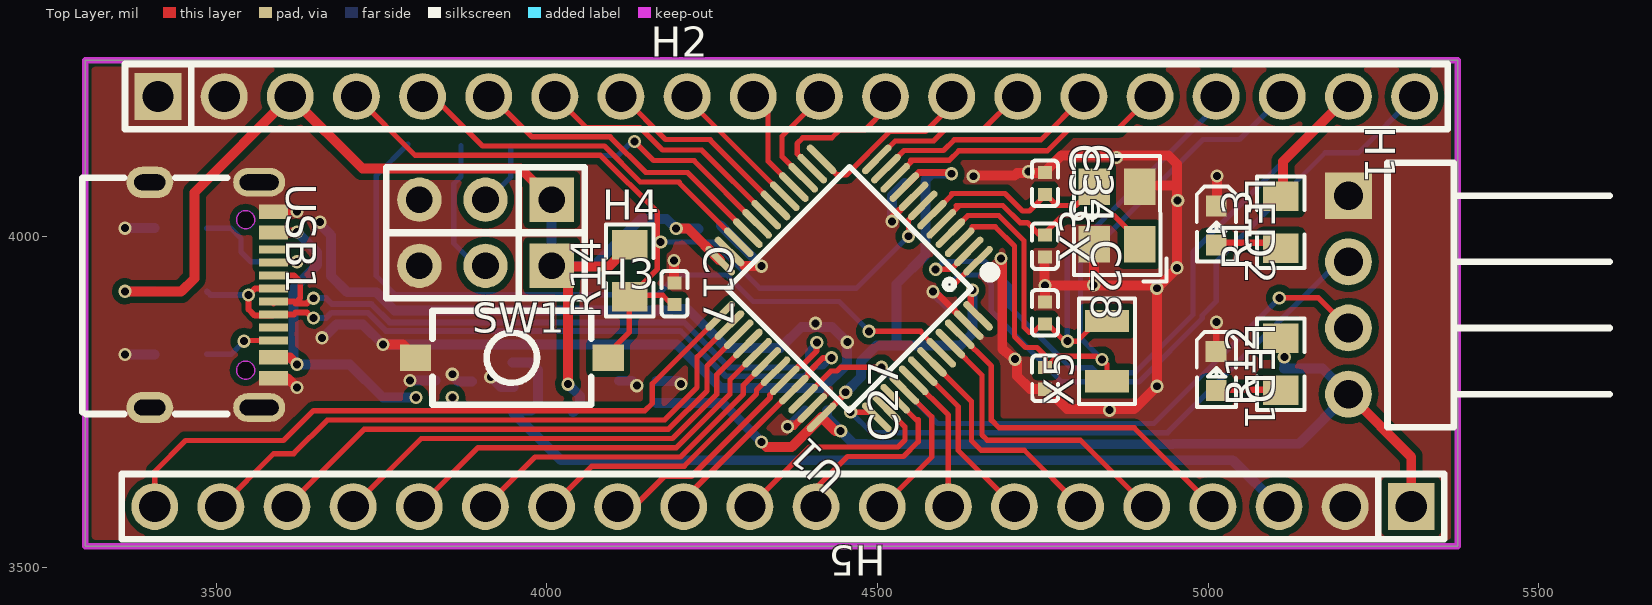
[diagram p0: Top Layer view]
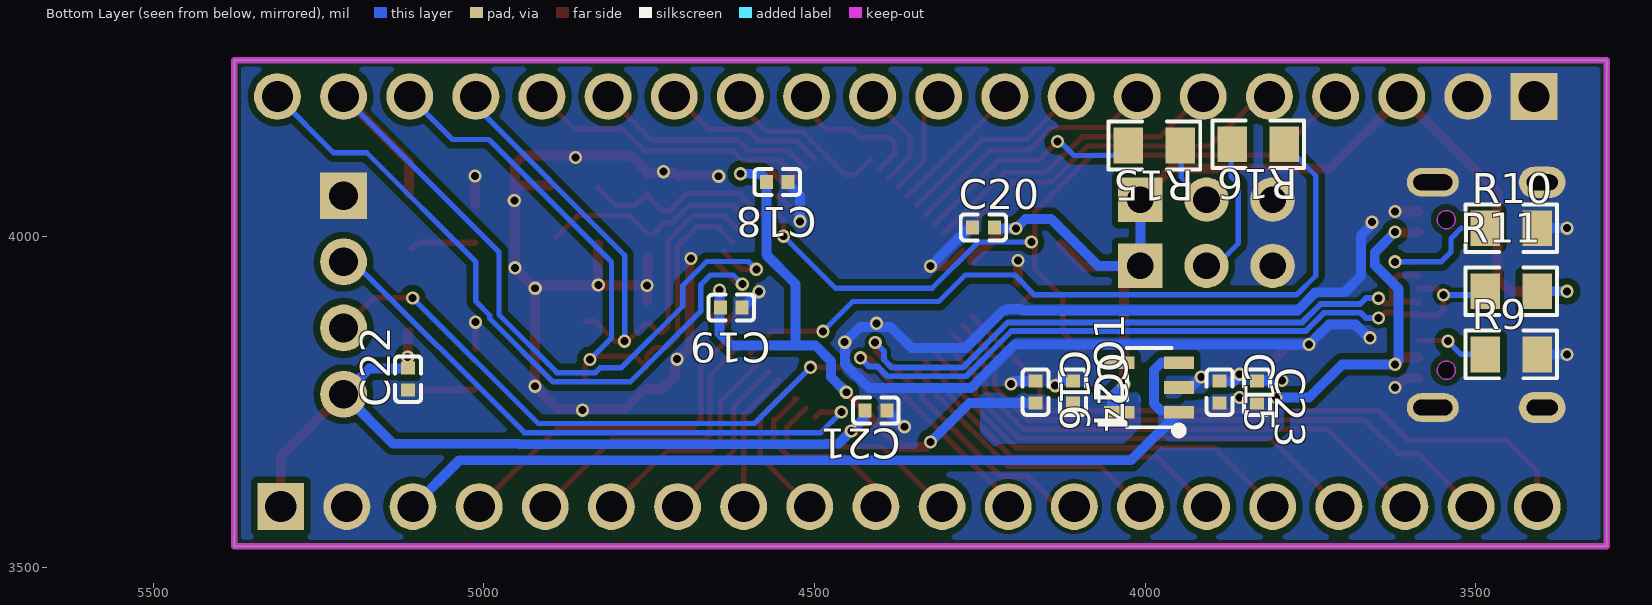
[diagram p1: Bottom Layer view, seen from below]
# Altium PCB MISC51884.pcbdoc
Units mil, origin at the board's own origin, x right, y up, seen from the top; angles counter-clockwise.
Board outline 2075 x 735 mil, 2 copper layers (Top Layer, Bottom Layer), stack 62.205 mil thick; 35 components, 49 nets, 175 pads, 64 vias.

## Layer stack, top to bottom
Top Solder Mask Layer: solder mask 0.394, Dk 3.3
Top Layer: signal copper 1.378
Dielectric1: surface 59.449, FR4, Dk 4.5
Bottom Layer: signal copper 1.378
Bottom Solder Mask Layer: solder mask 0.394, Dk 3.3

## Board outline
3301.94,4266.99 3301.94,3531.99 5376.94,3531.99 5376.94,4266.99

## Design rules (kind name [scope] priority, off if disabled: settings)
BoardOutlineClearance copperThickness2oz_1 [All] p2 off: genericclearance=7.99 ignorepadtopadclearanceinfootprint=FALSE except(0: Arc-SplitContinuation Track-SplitContinuation SMDPad-SplitContinuation THPad-SplitContinuation Via-SplitContinuation Fill-SplitContinuation Region-SplitContinuation Poly-SplitContinuation Text-SplitContinuation Hole-SplitContinuation; 5.98: Arc-CutoutEdge SMDPad-CutoutEdge THPad-CutoutEdge Via-CutoutEdge Fill-CutoutEdge Region-CutoutEdge Text-CutoutEdge; 6.93: Hole-OutlineEdge Hole-CutoutEdge; 10: Poly-OutlineEdge Poly-CutoutEdge; 11.81: Arc-OutlineEdge Track-OutlineEdge SMDPad-OutlineEdge THPad-OutlineEdge Via-OutlineEdge Fill-OutlineEdge Region-OutlineEdge Text-OutlineEdge Track-CutoutEdge)
BoardOutlineClearance safeClearance1_1 [All] p4: genericclearance=6 ignorepadtopadclearanceinfootprint=FALSE except(0: Arc-SplitContinuation Track-SplitContinuation SMDPad-SplitContinuation THPad-SplitContinuation Via-SplitContinuation Fill-SplitContinuation Region-SplitContinuation Poly-SplitContinuation Text-SplitContinuation Hole-SplitContinuation; 6: Arc-CutoutEdge Track-CutoutEdge SMDPad-CutoutEdge THPad-CutoutEdge Via-CutoutEdge Fill-CutoutEdge Region-CutoutEdge Text-CutoutEdge Hole-CutoutEdge; 10: Poly-OutlineEdge Poly-CutoutEdge; 11.8: Arc-OutlineEdge Track-OutlineEdge SMDPad-OutlineEdge THPad-OutlineEdge Via-OutlineEdge Fill-OutlineEdge Region-OutlineEdge Text-OutlineEdge Hole-OutlineEdge)
BoardOutlineClearance copperThickness1oz_1 [All] p6: genericclearance=6 ignorepadtopadclearanceinfootprint=FALSE except(0: Arc-SplitContinuation Track-SplitContinuation SMDPad-SplitContinuation THPad-SplitContinuation Via-SplitContinuation Fill-SplitContinuation Region-SplitContinuation Poly-SplitContinuation Text-SplitContinuation Hole-SplitContinuation; 6: Track-CutoutEdge SMDPad-CutoutEdge THPad-CutoutEdge Via-CutoutEdge Text-CutoutEdge; 6.93: Hole-OutlineEdge Hole-CutoutEdge; 10: Poly-OutlineEdge Poly-CutoutEdge; 11.8: Arc-OutlineEdge Track-OutlineEdge SMDPad-OutlineEdge THPad-OutlineEdge Via-OutlineEdge Fill-OutlineEdge Region-OutlineEdge Text-OutlineEdge Fill-CutoutEdge Region-CutoutEdge; 11.81: Arc-CutoutEdge)
Clearance copperThickness2oz [All] p1 off: gap=7.99 ignorepadtopadclearanceinfootprint=FALSE except(5.98: SMDPad-Track SMDPad-SMDPad THPad-Track SMDPad-THPad THPad-THPad Track-Via SMDPad-Via THPad-Via Via-Via Fill-Track Region-Track Fill-SMDPad Region-SMDPad Fill-THPad Region-THPad Fill-Via Region-Via Fill-Fill Fill-Region Region-Region Arc-Track Arc-SMDPad Arc-THPad Arc-Via Fill-Arc Region-Arc Arc-Arc Text-Track SMDPad-Text Text-THPad Text-Via Fill-Text Region-Text Arc-Text Text-Text; 6.93: Hole-Track Hole-SMDPad Hole-THPad Hole-Via Fill-Hole Region-Hole Hole-Arc Hole-Text; 10: Poly-Track Poly-SMDPad Poly-THPad Poly-Via Poly-Fill Poly-Region Poly-Poly Poly-Arc Poly-Text Poly-Hole)
Clearance safeClearance1 [(InNet('USB_D-_PA11')) vs (InNet('GND'))] p3: gap=6 ignorepadtopadclearanceinfootprint=FALSE except(10: Poly-Arc Poly-Text Poly-Hole)
Clearance copperThickness1oz [All] p5: gap=6 ignorepadtopadclearanceinfootprint=FALSE except(5.98: SMDPad-Track SMDPad-SMDPad THPad-Track SMDPad-THPad THPad-THPad Track-Via SMDPad-Via THPad-Via Via-Via Fill-SMDPad Region-SMDPad Fill-THPad Region-THPad Fill-Via Region-Via Fill-Fill Fill-Region Region-Region; 6.93: Hole-Track Hole-SMDPad Hole-THPad Hole-Via Fill-Hole Region-Hole Hole-Arc Hole-Text; 10: Poly-Track Poly-SMDPad Poly-THPad Poly-Via Poly-Fill Poly-Region Poly-Poly Poly-Arc Poly-Text Poly-Hole; 11.8: Fill-Track Region-Track)
DiffPairsRouting differentialPair [All] p1: maxlimit=6 minlimit=6 mostfreqgap=6 toplayer_minwidth=5 toplayer_prefwidth=9 toplayer_maxwidth=100 toplayer_mingap=4 toplayer_prefgap=5 toplayer_maxgap=5 bottomlayer_minwidth=5 bottomlayer_prefwidth=9 bottomlayer_maxwidth=100 bottomlayer_mingap=4 bottomlayer_prefgap=5 bottomlayer_maxgap=5 maxuncoupledlength=1000
HoleToHoleClearance otherClearance [All] p1: gap=11.81 allowstackedmicrovias=TRUE
Length netLength [All] p1: minlimit=0 maxlimit=0
MatchedLengths netLengthTolerance [All] p1: tolerance=1000
PasteMaskExpansion pasteMaskExpansion [All] p1: expansion=0
PlaneConnect innerPlane [All] p1: planeconnectstyle=Relief reliefexpansion=20 reliefentries=4 reliefconductorwidth=10 reliefairgap=10
PolygonConnect "copperRegion_Top Layer" [(InNet('GND')) And OnLayer('Top Layer')] p1: connectstyle=Direct reliefconductorwidth=10 reliefentries=4 polygonreliefangle="90 Angle" airgapwidth=10 via.connectstyle=Relief via.reliefconductorwidth=10 via.reliefentries=4 via.polygonreliefangle="90 Angle" via.airgapwidth=10
PolygonConnect "copperRegion_Bottom Layer" [(InNet('GND')) And OnLayer('Bottom Layer')] p2: connectstyle=Direct reliefconductorwidth=10 reliefentries=4 polygonreliefangle="90 Angle" airgapwidth=10 via.connectstyle=Relief via.reliefconductorwidth=10 via.reliefentries=4 via.polygonreliefangle="90 Angle" via.airgapwidth=10
PolygonConnect copperRegion [(InNet('GND'))] p3: connectstyle=Direct reliefconductorwidth=10 reliefentries=4 polygonreliefangle="90 Angle" airgapwidth=10 via.connectstyle=Relief via.reliefconductorwidth=10 via.reliefentries=4 via.polygonreliefangle="90 Angle" via.airgapwidth=10
RoutingVias viaSize [All] p1: holewidth=12 width=20 viastyle="Through Hole" minholewidth=11.81 minwidth=19.68 maxholewidth=248.03 maxwidth=393.7
SolderMaskExpansion solderMaskExpansion [IsVia] p1: expansion=-1000 istentingtop=TRUE
SolderMaskExpansion solderMaskExpansion [All] p2: expansion=2 istentingtop=FALSE
Width pwr [(InNet('+5V') OR InNet('GND') OR InNet('3V3'))] p1: maxlimit=10 minlimit=10 preferedwidth=10 toplayer_minwidth=5 toplayer_maxwidth=100 toplayer_prefwidth=15 bottomlayer_minwidth=5 bottomlayer_maxwidth=100 bottomlayer_prefwidth=15
Width copperThickness1oz_2 [All] p2: maxlimit=10 minlimit=10 preferedwidth=10 toplayer_minwidth=5 toplayer_maxwidth=100 toplayer_prefwidth=8 bottomlayer_minwidth=5 bottomlayer_maxwidth=100 bottomlayer_prefwidth=8

## Components (designator, comment, footprint, x,y, rotation, side; value= is the part's Value field where it differs from the comment)
C15 "100nF" C0402 3887.18,3765.13 r270 bottom
C16 "100nF" C0402 4165.39,3765.13 r270 bottom
C17 "100nF" C0402 4192.92,3913.82 r270 top
C18 "100nF" C0402 4556.15,4082.72 r0 bottom
C19 "100nF" C0402 4625.75,3892.7 r0 bottom
C20 "100nF" C0402 4244.28,4014.21 r180 bottom
C21 "100nF" C0402 4406.94,3736.99 r0 bottom
C22 "100nF" C0402 5114.29,3784.59 r90 bottom
C23 "1uF" C0402 3830.97,3765.13 r270 bottom
C24 "1uF" C0402 4109.18,3765.13 r270 bottom
C27 "12pF" C0402 4753.42,3785.9 r90 top
C28 "12pF" C0402 4752.88,3884.91 r270 top
C33 "12pF" C0402 4752.85,4080.7 r270 top
C34 "12pF" C0402 4752.85,3985.84 r270 top
H1 "DZ254W-11-04-65" HDR-TH_4P-P2.54-H-M-W10.3 5211.94,3911.99 r270 top
H2 "2.54-1*20P直针" HDR-TH_20P-P2.54-V-M-1 4361.94,4211.99 r0 top
H3 "PZ254V-11-03P" HDR-TH_3P-P2.54-V-M_PZ254V-11-03P 3907.09,3955.98 r180 top
H4 "PZ254V-11-03P" HDR-TH_3P-P2.54-V-M_PZ254V-11-03P 3907.09,4055.98 r180 top
H5 "2.54-1*20P直针" HDR-TH_20P-P2.54-V-M-1 4356.94,3591.99 r180 top
LDO1 "ME6211C33M5G-N" SOT-23-5_L3.0-W1.7-P0.95-LS2.8-BL 3993.82,3771.99 r90 bottom
LED1 "NCD0603R1" LED0603-RD_RED 5011.94,3796.99 r270 top
LED2 "NCD0603B1" LED0603-RD 5011.94,4016.99 r270 top
R9 "5.1kΩ" R0805 3446.31,3822.08 r180 bottom
R10 "5.1kΩ" R0805 3446.31,4012.89 r180 bottom
R11 "1.5kΩ" R0805 3446.31,3917.48 r180 bottom
R12 "1kΩ" R0805 5109.57,3807.13 r90 top
R13 "1kΩ" R0805 5109.57,4021.85 r90 top
R14 "10kΩ" R0805 4125.3,3948.81 r90 top
R15 "10kΩ" R0805 3985.86,4138.03 r0 bottom
R16 "10kΩ" R0805 3829.01,4139.92 r0 bottom
SW1 "TS-1101-B-W" KEY-SMD_2P-L6.0-W3.6-P7.4-LS8.0-L 3946.94,3816.99 r0 top
U1 "STM32F103C8T6" LQFP-48_L7.0-W7.0-P0.50-LS9.0-BL 4456.94,3921.99 r135 top
USB1 "TYPE-C 16PIN 2MD(073)" USB-C-SMD_TYPE-C-6PIN-2MD-073 3493.04,3911.99 r270 top
X3 "8MHz" CRYSTAL-SMD_4P-L3.2-W2.5-BL-1 4861.94,4031.99 r90 top
X5 "32.768kHz" OSC-SMD_L3.2-W1.5 4846.94,3826.99 r90 top

## Footprints (in the part's own frame and the unit in brackets; to place one, negate y for a bottom-side part, rotate by r counter-clockwise, add the part's x,y. Pads: shape width x height; smd on the part's side, far side on the other; paste and mask are expansions set on the pad)
C0402 [mm]
  rect 0.5x0.54 smd: 1(-0.42,0) 2(0.42,0)
  silkscreen extent -0.87,-0.5 0.87,0.5
CRYSTAL-SMD_4P-L3.2-W2.5-BL-1 [mm]
  rect 1.4x1.2 smd: 1(-1.1,-0.875) 2(1.1,-0.875) 3(1.1,0.875) 4(-1.1,0.875)
  silkscreen extent -2.54,-1.9 2.29,1.65
HDR-TH_3P-P2.54-V-M_PZ254V-11-03P [mm]
  rect 1.7x1.7 hole 1.02: 1(-2.54,0)
  round 1.7 hole 1.02: 2(0,0) 3(2.54,0)
  silkscreen extent -3.81,-1.25 3.81,1.25
HDR-TH_4P-P2.54-H-M-W10.3 [mm]
  rect 1.8x1.8 hole 1.1: 1(-3.81,0)
  round 1.8 hole 1.1: 2(-1.27,0) 3(1.27,0) 4(3.81,0)
  silkscreen extent -5.08,1.5 5.08,10.04
HDR-TH_20P-P2.54-V-M-1 [mm]
  rect 1.8x1.8 hole 1.2: 1(-24.13,0)
  round 1.8 hole 1.2: 2(-21.59,0) 3(-19.05,0) 4(-16.51,0) 5(-13.97,0) 6(-11.43,0) 7(-8.89,0) 8(-6.35,0) 9(-3.81,0) 10(-1.27,0) 11(1.27,0) 12(3.81,0) 13(6.35,0) 14(8.89,0) 15(11.43,0) 16(13.97,0) 17(16.51,0) 18(19.05,0) 19(21.59,0) 20(24.13,0)
  silkscreen extent -25.4,-1.25 25.4,1.25
KEY-SMD_2P-L6.0-W3.6-P7.4-LS8.0-L [mm]
  rect 1.2x1 smd: 1(-3.7,0) 2(3.7,0)
  silkscreen extent -3.05,-1.8 3.05,1.8
LED0603-RD [mm]
  rect 0.8x0.8 smd: 1(-0.749,0) 2(0.749,0)
  silkscreen extent -1.49,-0.75 1.39,0.76
LED0603-RD_RED [mm]
  rect 0.8x0.8 smd: 1(-0.749,-0.003) 2(0.749,0.003)
  silkscreen extent -1.49,-0.75 1.39,0.76
LQFP-48_L7.0-W7.0-P0.50-LS9.0-BL [mm]
  oval 0.27x1.5 smd paste+0 mask+0.05: 1(-2.75,-4.25) 2(-2.25,-4.25) 3(-1.75,-4.25) 4(-1.25,-4.25) 5(-0.75,-4.25) 6(-0.25,-4.25) 7(0.25,-4.25) 8(0.75,-4.25) 9(1.25,-4.25) 10(1.75,-4.25) 11(2.25,-4.25) 12(2.75,-4.25) 25(2.75,4.25) 26(2.25,4.25) 27(1.75,4.25) 28(1.25,4.25) 29(0.75,4.25) 30(0.25,4.25) 31(-0.25,4.25) 32(-0.75,4.25) 33(-1.25,4.25) 34(-1.75,4.25) 35(-2.25,4.25) 36(-2.75,4.25)
  oval 1.5x0.27 smd paste+0 mask+0.05: 13(4.25,-2.75) 14(4.25,-2.25) 15(4.25,-1.75) 16(4.25,-1.25) 17(4.25,-0.75) 18(4.25,-0.25) 19(4.25,0.25) 20(4.25,0.75) 21(4.25,1.25) 22(4.25,1.75) 23(4.25,2.25) 24(4.25,2.75) 37(-4.25,2.75) 38(-4.25,2.25) 39(-4.25,1.75) 40(-4.25,1.25) 41(-4.25,0.75) 42(-4.25,0.25) 43(-4.25,-0.25) 44(-4.25,-0.75) 45(-4.25,-1.25) 46(-4.25,-1.75) 47(-4.25,-2.25) 48(-4.25,-2.75)
  silkscreen extent -3.59,-4.46 3.3,3.34
OSC-SMD_L3.2-W1.5 [mm]
  rect 0.85x1.7 smd: 1(-1.155,0) 2(1.155,0)
  silkscreen extent -2.03,-1.08 2.03,1.08
R0805 [mm]
  rect 1.133x1.377 smd paste-100 mask+0.051: 1(-1,0) 2(1,0)
  silkscreen extent -1.76,-0.92 1.76,0.92
SOT-23-5_L3.0-W1.7-P0.95-LS2.8-BL [mm]
  rect 0.49x1.157 smd: 1(-0.95,-1.154) 2(0,-1.154) 3(0.95,-1.154)
  rect 0.49x1.175 smd: 4(0.95,1.154) 5(-0.95,1.154)
  silkscreen extent -1.8,-1.29 1.53,0.85
USB-C-SMD_TYPE-C-6PIN-2MD-073 [mm]
  rect 0.55x1.1 smd paste-100 mask+0.05: 1(-3.2,2.375) 2(-2.4,2.375) 11(2.4,2.375) 12(3.2,2.375)
  rect 0.3x1.1 smd paste-100 mask+0.05: 3(-1.75,2.375) 4(-1.25,2.375) 5(-0.75,2.375) 6(-0.25,2.375) 7(0.25,2.375) 8(0.75,2.375) 9(1.25,2.375) 10(1.75,2.375)
  oval 1.2x1.8 hole 0.6 slot 1.2 at 90 deg paste+0 mask+0.05: 13(-4.325,-2.375) 14(4.325,-2.375)
  oval 1.1x2 hole 0.6 slot 1.5 at 90 deg paste+0 mask+0.05: 13(-4.325,1.825) 14(4.325,1.825)
  Board Outline Layer circle w0.003: c-2.89,1.305 r0.35
  Board Outline Layer circle w0.003: c2.89,1.305 r0.35
  Board Outline Layer region: -2.89,1.655 -2.738,1.62 -2.616,1.523 -2.549,1.383 -2.549,1.227 -2.616,1.087 -2.738,0.99 -2.89,0.955 -2.89,0.955 -3.042,0.99 -3.164,1.087 -3.231,1.227 -3.231,1.383 -3.164,1.523 -3.042,1.62 -2.89,1.655
  Board Outline Layer region: -2.89,1.655 -2.812,1.646 -2.738,1.62 -2.672,1.579 -2.616,1.523 -2.575,1.457 -2.549,1.383 -2.54,1.305 -2.549,1.227 -2.575,1.153 -2.616,1.087 -2.672,1.031 -2.738,0.99 -2.812,0.964 -2.89,0.955 -2.968,0.964 -3.042,0.99 -3.108,1.031 -3.164,1.087 -3.205,1.153 -3.231,1.227 -3.24,1.305 -3.231,1.383 -3.205,1.457 -3.164,1.523 -3.108,1.579 -3.042,1.62 -2.968,1.646
  Board Outline Layer region: 2.89,1.655 3.042,1.62 3.164,1.523 3.231,1.383 3.231,1.227 3.164,1.087 3.042,0.99 2.89,0.955 2.89,0.955 2.738,0.99 2.616,1.087 2.549,1.227 2.549,1.383 2.616,1.523 2.738,1.62 2.89,1.655
  Board Outline Layer region: 2.89,1.655 2.968,1.646 3.042,1.62 3.108,1.579 3.164,1.523 3.205,1.457 3.231,1.383 3.24,1.305 3.231,1.227 3.205,1.153 3.164,1.087 3.108,1.031 3.042,0.99 2.968,0.964 2.89,0.955 2.812,0.964 2.738,0.99 2.672,1.031 2.616,1.087 2.575,1.153 2.549,1.227 2.54,1.305 2.549,1.383 2.575,1.457 2.616,1.523 2.672,1.579 2.738,1.62 2.812,1.646
  Multi-Layer board cut-out: -2.89,1.655 -2.738,1.62 -2.616,1.523 -2.549,1.383 -2.549,1.227 -2.616,1.087 -2.738,0.99 -2.89,0.955 -2.89,0.955 -3.042,0.99 -3.164,1.087 -3.231,1.227 -3.231,1.383 -3.164,1.523 -3.042,1.62 -2.89,1.655
  Multi-Layer board cut-out: 2.89,1.655 3.042,1.62 3.164,1.523 3.231,1.383 3.231,1.227 3.164,1.087 3.042,0.99 2.89,0.955 2.89,0.955 2.738,0.99 2.616,1.087 2.549,1.227 2.549,1.383 2.616,1.523 2.738,1.62 2.89,1.655
  silkscreen extent -4.5,-4.97 4.57,0.6

## Via types
v1: diameter 20, hole 12, Top Layer to Bottom Layer, 64 vias

## Nets (pads, with @x,y where several pads share a name; then routed paths per layer and width w, separated by ;. In a path a pad name is that pad's centre, name@x,y a point inside that pad or via, vN(x,y) a via of type N, cw(c..) or ccw(c..) an arc to the next point about the centre after c; other vN are vias at no path point)
3V3: C16.2 C18.2 C19.2 C20.2 C21.2 C22.2 C24.2 H1.4 H2.3 H3.1 H4.1 H5.1 LDO1.5 R11.2 R12.2 R14.2 U1.9 U1.24 U1.36 U1.48 | length 4121
  Top Layer w10: U1.36 v1@4451.7,3763.64 ; U1.9 4562.45,4097.09 ; 4562.22,4097.09 4562.45,4097.09 ; v1(4611.86,4095.24) 4610.01,4097.09 4562.45,4097.09 ; v1(4643.5,3919.17) 4641.01,3916.68 4641.01,3891.04 U1.48
  Top Layer w15: v1(3361.94,3917.48) 3362.43,3916.99 3446.94,3916.99 3466.94,3936.99 3466.94,4066.99 H2.3 3721.01,4102.93 3960.14,4102.93 H4.1 ; H3.1 4031.94,3931.12 v1(4031.94,3776.99) ; H3.1@4010.18,3955.18 4093.96,3955.18 R14.2@4126.94,3988.16 ; v1(4195.4,4012.55) 4213.27,4012.55 U1.24 ; v1(4324.44,3689.49) 4331.94,3681.99 4370.06,3681.99 U1.36 4436.01,3706.3 v1(4444.17,3706.3) ; R12.2@5113.38,3856.18 5114.92,3854.64 v1(5114.92,3818.06) ; H1.4 5306.94,3667 H5.1
  Bottom Layer w15: v1(3361.94,3917.48) R11.2 ; H4.1 H3.1 4070.93,3955.98 4141.94,4026.99 4180.96,4026.99 v1(4195.4,4012.55) 4228.31,4012.55 C20.2@4229.39,4011.47 ; v1(4031.94,3776.99) 4049.84,3759.09 4049.84,3745.2 LDO1.5 ; C16.2 4265.34,3748.59 v1(4324.44,3689.49) ; C21.2 4423.48,3726.99 v1(4444.17,3706.3) 4463.48,3686.99 4482.23,3686.99 4483.05,3686.18 4945.87,3686.18 4946.69,3686.99 5136.94,3686.99 H1.4@5211.68,3761.73 ; v1(4451.7,3764.78) 4474.82,3787.9 4474.82,3811.66 4498.54,3835.39 4528.57,3835.39 ; C18.2 4572.69,3972.74 4528.57,3928.62 4528.57,3835.39 ; C18.2@4573.09,4087 4581.34,4095.24 v1(4611.86,4095.24) ; v1(4643.5,3919.17) C19.2@4643.5,3894.17 ; C19.2@4643.7,3893.97 C19.2@4643.5,3894.17 ; C22.2@5114.15,3800.69 5172.73,3800.69 H1.4@5211.68,3761.73 ; C22.2@5114.92,3805.31 v1(5114.92,3818.06) ; H1.4 H1.4@5211.68,3761.73 ; 4528.57,3835.39 4625.33,3835.39 4643.5,3853.56 C19.2@4643.5,3894.17
$1N141: R9.1 USB1.10 | length 109.6
  Top Layer w8: v1(3541.94,3841.99) 3543.04,3843.09 USB1.10
  Bottom Layer w8: R9.1 3522.02,3822.08 v1(3541.94,3841.99)
$1N146: R10.1 USB1.4 | length 205
  Top Layer w8: USB1.4 3587.34,3961.99 v1(3621.94,3961.99)
  Bottom Layer w8: R10.1 3521.94,4012.89 3537.39,3997.44 3537.39,3976.99 3552.39,3961.99 v1(3621.94,3961.99)
$1N157: LED1.2 R12.1 | length 96.1
  Top Layer w10: LED1.2@5015.31,3768.32 5107.02,3768.32 R12.1@5110.11,3771.4
$1N159: LED2.2 R13.1 | length 98.3
  Top Layer w10: LED2.2@5013,3990.86 5099.32,3990.86 R13.1@5107.79,3982.38
$1N169: H3.2 R16.2 | length 216
  Bottom Layer w8: R16.2@3870.17,4137.87 3870.17,4091.2 3859.01,4080.04 3859.01,3989.74 3896.55,3952.2 H3.2@3906.7,3952.2
$1N174: H4.2 R15.1 | length 98.3
  Bottom Layer w8: H4.2@3908.72,4053.66 3945.25,4090.19 R15.1@3945.25,4136.86
+5V: C15.2 C23.2 H5.3 LDO1.1 LDO1.3 USB1.2 USB1.11 | length 1856.5
  Top Layer w15: USB1.11 3611.43,3817.5 v1(3621.92,3807.01) ; USB1.2 3621.43,4006.48 v1(3621.94,4006.99)
  Bottom Layer w15: v1(3621.94,4006.99) 3652.63,3976.3 3652.63,3956.99 3616.94,3921.3 3616.94,3811.99 v1(3621.92,3807.01) 3701.92,3807.01 3751.94,3756.99 v1(3801.94,3756.99) ; LDO1.3@3947.88,3809.85 3975.29,3809.85 3986.58,3798.56 3986.58,3747.5 3975.97,3736.9 3952.33,3736.9 LDO1.1@3952.18,3736.76 ; LDO1.1 4021,3661.99 5036.94,3661.99 H5.3
  other v1: 3856.94,3756.99
BOOT0: R16.1 U1.44 | length 1147.8
  Top Layer w8: v1(4486.94,3856.99) 4565.64,3856.99 ; 4563.7,3856.99 U1.44
  Bottom Layer w8: R16.1 3741.94,4092.22 3741.94,3941.04 3770.83,3912.14 4167.09,3912.14 4196.94,3941.99 4271.94,3941.99 4311.94,3901.99 4441.94,3901.99 v1(4486.94,3856.99)
BOOT1: R15.2 U1.20 | length 347
  Top Layer w8: v1(4132.44,4144.03) 4161.3,4115.16 4222.94,4115.16 ; 4222,4115.16 U1.20
  Bottom Layer w8: R15.2@4031.49,4122.65 4107.59,4122.65 v1@4130.93,4145.99
GND: C15.1 C16.1 C17.1 C18.1 C19.1 C20.1 C21.1 C22.1 C23.1 C24.1 C27.1 C28.1 C33.1 C34.2 H1.1 H2.1 H2.2 H3.3 H4.3 H5.2 LDO1.2 LED1.1 LED2.1 R9.2 R10.2 SW1.1 U1.8 U1.23 U1.35 U1.47 USB1.1 USB1.12 USB1.13 USB1.14 X3.2 X3.4 | length 4271.5
  Top Layer w10: U1.23 4298.14,3955.52 ; v1@4364.3,3712.81 v1@4373.54,3712.81 ; v1@4373.03,3712.81 U1.35 ; v1@4521.86,4023.23 v1@4521.86,4031.08 ; v1@4521.86,4028.67 U1.8 ; v1@4583.15,3917.71 v1@4586.39,3917.71 ; v1@4586.49,3917.71 U1.47 ; LED1.1@5012.23,3830.74 v1(5012.23,3870.82)
  Top Layer w15: USB1.12 3607.92,3786.01 v1(3621.94,3771.99) ; USB1.1 v1(3621.94,4037.98) ; v1(3751.94,3836.99) 3782.47,3836.99 SW1.1@3801.31,3818.15 ; C17.1@4192,3931.79 v1(4192,3963.87) ; 4298.56,3955.52 v1@4324.45,3955.52 ; v1@4645.01,4092.55 4707.28,4092.55 4710.98,4096.24 C33.1@4752.9,4096.24 ; v1(4686.7,3966.89) 4688.47,3965.13 4688.47,3830.37 v1@4708.9,3813.81 ; v1(4707.91,3814.81) v1@4708.9,3813.81 ; C34.2@4752.52,3966.86 4752.52,3927.67 v1@4753.4,3926.79 ; C28.1@4752.96,3903 v1(4752.96,3926.34) v1@4926.93,3926.34 ; C33.1@4753.52,4098.71 4777.7,4122.89 4939.95,4122.89 4952.9,4109.94 v1@4952.9,3953.02 ; C27.1@4754.84,3770.03 4730.56,3770.03 4710.99,3789.61 4710.99,3811.73 v1@4708.9,3813.81 ; C27.1@4759.16,3766.79 4786.54,3739.41 4887.96,3739.41 v1(4922.43,3773.88) 4922.21,3774.1 v1(4922.21,3922.08) ; v1@4827.03,3927.54 X3.4@4827.03,3988.24 ; X3.2@4899.86,4077.25 4947.06,4077.25 4952.46,4082.65 ; v1@4922.66,3922.07 v1@4926.93,3926.34 ; v1@4953.48,3951.58 4952.16,3951.58 v1@4926.93,3926.34 ; LED2.1@5013,4049.43 v1(5013,4091.82)
  Bottom Layer w15: v1(3361.94,3822.08) R9.2 ; v1(3361.94,4012.89) R10.2 ; v1@3654.92,4020.85 3673.63,4002.14 3673.63,3940.49 3698.13,3915.99 3742.24,3915.99 3769.71,3888.52 4186.41,3888.52 4188.6,3890.7 4208.23,3890.7 4210.41,3888.52 4214.71,3888.52 4271.24,3831.99 4353.18,3831.99 4384.69,3863.5 4405.9,3863.5 v1(4405.9,3869) 4411.4,3863.5 4431.19,3863.5 v1(4454.21,3840.48) 4453.82,3840.09 4453.82,3807.15 4417.65,3770.99 4262.94,3770.99 4196.94,3836.99 v1(3751.94,3836.99) 3721.94,3866.99 3681.48,3866.99 v1@3662.43,3847.94 ; v1(3793.01,3782.48) 3793.32,3782.79 C23.1@3831.86,3782.79 ; v1@3856.52,3790.63 3865.9,3781.25 C15.1@3886.73,3781.25 ; v1(3915,3787.74) 3930.42,3772.33 LDO1.2@3949.38,3772.33 ; C24.1@4108.79,3782.21 4128.52,3782.21 v1(4135.92,3774.81) ; C16.1@4165.33,3781.65 4198.24,3781.65 v1(4202.55,3777.34) ; C20.1@4262.86,4016.98 v1(4324.36,3955.48) ; v1(4363.61,3712.68) 4366.09,3712.68 C21.1 ; v1(4521.61,4023.26) 4521.61,4062.34 C18.1@4540.57,4081.3 ; v1(4583.66,3916.86) 4583.97,3916.86 C19.1@4608.02,3892.82
  other v1: 4850.64,3737.66 3856.94,3791.99 3659.74,3847.17 4826.7,3926.85 4952.82,3953.02 3656.94,4021.99 4953.7,4054.75 4644.7,4091.47 4727.99,4098.35 4861.32,4119.93
NRST: C17.2 H2.4 R14.1 SW1.2 U1.7 | length 1324.1
  Top Layer w8: H2.4 3800.86,4123.07 4081.1,4123.07 4166.94,4037.23 4166.94,3951.08 R14.1@4127.37,3911.51 ; SW1.2@4093.96,3825.06 4124.26,3855.36 R14.1@4124.26,3909.44 ; R14.1 R14.1@4127.37,3911.51 ; C17.2@4185.76,3900.81 4175.06,3911.51 R14.1@4127.37,3911.51 ; v1(4546.73,4000.66) 4546.73,4025.7 U1.7
  Bottom Layer w8: v1(4171.94,3991.99) 4251.94,3991.99 4321.94,3921.99 4468.06,3921.99 v1(4546.73,4000.66)
OSC32_IN: C27.2 H2.18 U1.3 X5.1 | length 1012.6
  Top Layer w8: U1.3 4647.52,4015.14 ; 4642.72,4015.14 4677.79,4015.14 4706.86,3986.06 4706.86,3849.32 4723.66,3832.52 4740.91,3832.52 4753.85,3819.57 C27.2@4753.85,3801.77 ; C27.2@4754.33,3802.61 4770.9,3819.18 v1@4830.94,3819.18 ; v1(4839.44,3814.49) 4846.94,3806.99 X5.1
  Bottom Layer w8: v1(4839.44,3814.49) 4806.92,3847.01 4806.92,3850.27 4806.71,3850.48 4806.71,3961.76 4991.94,4146.99 5046.94,4146.99 H2.18
OSC32_OUT: C28.2 H2.17 U1.4 X5.2 | length 881.7
  Top Layer w8: U1.4 4636.47,4031.93 ; 4636.89,4031.93 4683.15,4031.93 4721.24,3993.84 4721.24,3863.11 4729.24,3855.11 4735.35,3855.11 C28.2@4749.91,3869.68 ; C28.2@4756.33,3868.5 v1@4784.39,3840.45 ; v1(4786.94,3841.99) 4801.94,3841.99 4832.41,3872.46 X5.2
  Bottom Layer w8: v1(4786.94,3841.99) 4786.94,3971.99 5011.94,4196.99 H2.17
OSC_IN: C34.1 U1.5 X3.1 | length 349.6
  Top Layer w8: U1.5 4623.81,4047.1 ; 4619.01,4047.1 4689.3,4047.1 4715.19,4021.21 4726.51,4021.21 4744.31,4003.4 C34.1@4748.49,4003.4 ; C34.1@4752.4,4005.02 4779.38,4032 4857.6,4032 X3.1@4890.51,3999.09
OSC_OUT: C33.2 U1.6 X3.3 | length 302.5
  Top Layer w8: U1.6 4614.31,4065.45 ; 4612.14,4065.45 4692.52,4065.45 4718.96,4039.01 4729.75,4039.01 C33.2@4754.56,4063.83 ; C33.2@4753.48,4064.91 C33.2@4754.56,4063.83 ; X3.3@4827.93,4075.16 4799.88,4047.1 4771.29,4047.1 C33.2@4754.56,4063.83
PA0: H2.16 U1.10 | length 438.1
  Top Layer w8: U1.10 4553.28,4115.77 ; 4550.3,4115.77 4608.57,4115.77 4622.86,4130.06 4756.93,4130.06 4790.11,4163.24 4863.75,4163.24 H2.16@4911.22,4210.72
PA1: H2.15 U1.11 | length 344.7
  Top Layer w8: U1.11 4540.02,4130.35 ; 4540.18,4130.35 4599.66,4130.35 4615.98,4146.67 4747.21,4146.67 H2.15@4812.35,4211.81
PA2: H2.14 U1.12 | length 248.1
  Top Layer w8: U1.12 4526.67,4144.84 ; 4530.29,4144.84 4584.78,4144.84 4602.01,4162.06 4659.46,4162.06 4708.83,4211.43 H2.14@4711.25,4211.43
PA3: H2.13 U1.13 | length 264.1
  Top Layer w8: U1.13@4415.12,4116.8 4438.32,4093.6 4452.89,4093.6 4518.32,4159.03 4572.27,4159.03 4613.25,4200.02 H2.13@4613.25,4212.29
PA4: H2.12 U1.14 | length 221.3
  Top Layer w8: 4378.36,4125.43 4378.36,4141.08 4386.99,4149.71 4430.69,4149.71 4442.56,4161.58 4480.86,4161.58 4512.69,4193.41 H2.12@4512.69,4210.67 ; 4378.36,4125.84 U1.14
PA5: H2.11 U1.15 | length 154.7
  Top Layer w8: 4355.3,4121.06 U1.15 ; 4355.3,4122.67 4355.3,4151.93 H2.11@4411.95,4208.58
PA6: H2.10 U1.16 | length 157.1
  Top Layer w8: H2.10@4314.44,4209.93 4334.26,4190.1 4334.26,4116.46 ; 4334.26,4114.26 U1.16
PA7: H2.9 U1.17 | length 210
  Top Layer w8: H2.9@4213.65,4207.04 U1.17 ; H2.9@4213.65,4207.33 H2.9@4213.65,4211.11
PA8: H5.16 U1.29 | length 619.9
  Top Layer w8: H5.16 3895.95,3681.01 4195.95,3681.01 4276.94,3761.99 4276.94,3783.75 U1.29
PA9/USART1_TX: H5.15 U1.30 | length 523.3
  Top Layer w8: H5.15 3981.95,3667.01 4201.75,3667.01 4296.94,3762.19 4296.94,3775.91 U1.30
PA10/USART1_RX: H5.14 U1.31 | length 426.8
  Top Layer w8: H5.14 4067.95,3653.01 4207.55,3653.01 4316.94,3762.39 4316.94,3768.08 U1.31
PA13/SWDIO: H1.3 U1.34 | length 976.9
  Top Layer w8: U1.34 4429.29,3796.9 4438.59,3796.9 4444.13,3802.45 v1(4505.79,3802.45) ; v1(5107.45,3907.5) 5166.43,3907.5 H1.3
  Bottom Layer w8: v1(4505.79,3802.45) 4590.56,3717.68 4917.62,3717.68 v1(5107.45,3907.5)
PA14/SWCLK: H1.2 U1.37 | length 915.2
  Top Layer w8: v1(4459.22,3734.75) 4491.06,3734.75 U1.37
  Bottom Layer w8: v1(4459.22,3734.75) 4490.3,3703.68 4938.62,3703.68 5196.94,3961.99 H1.2
PA15: H5.11 U1.38 | length 336.8
  Top Layer w8: H5.11 4396.86,3681.92 4530.58,3681.92 4541.44,3692.77 4541.44,3712.6 ; U1.38 4541.44,3712.22
PB0: H2.8 U1.18 | length 303.4
  Top Layer w8: H2.8@4111.45,4210.4 4116.18,4210.4 4179.43,4147.15 4247.41,4147.15 ; 4245.7,4147.15 U1.18
PB1: H2.7 U1.19 | length 391.2
  Top Layer w8: H2.7@4013.21,4208.5 4016.04,4208.5 4059.47,4165.07 4140.66,4165.07 4174.65,4131.08 4234.13,4131.08 ; 4233.93,4131.08 U1.19
PB3: H5.10 U1.39 | length 297.6
  Top Layer w8: H5.10 4406.94,3620.11 4454.58,3667.76 4539.08,3667.76 4561.26,3689.94 4561.26,3723.67 ; U1.39@4529.97,3754.96 U1.39 4561.26,3720.23
PB4: H5.9 U1.40 | length 225.4
  Top Layer w8: H5.9 4581.94,3666.99 4581.94,3727.67 ; U1.40 4581.94,3727.4
PB5: H5.8 U1.41 | length 211.5
  Top Layer w8: U1.41 4606.94,3730.23 ; H5.8 4606.94,3729.1
PB6: H5.7 U1.42 | length 261.5
  Top Layer w8: U1.42 4621.94,3743.08 ; 4621.94,3742.43 4621.94,3676.99 H5.7
PB7: H5.6 U1.43 | length 350.2
  Top Layer w8: U1.43 4641.94,3750.91 ; 4641.94,3751.02 4641.94,3691.54 4656.35,3677.13 4721.8,3677.13 H5.6
PB8: H5.5 U1.45 | length 450.3
  Top Layer w8: U1.45 4657.94,3790.58 ; 4657.94,3788.97 4657.94,3700.2 4665.94,3692.2 4806.73,3692.2 H5.5
PB9: H5.4 U1.46 | length 538.1
  Top Layer w8: U1.46 4671.94,3804.43 ; 4671.94,3803.83 4671.94,3722.64 4683.5,3711.08 4887.85,3711.08 H5.4
PB10: H2.6 U1.21 | length 477.4
  Top Layer w8: H2.6@3912.63,4212.21 3916.4,4212.21 3977.54,4151.07 4095.56,4151.07 4149.6,4097.02 4212.31,4097.02 ; 4212.85,4097.02 4212.31,4097.02 ; U1.21 4212.31,4097.02
PB11: H2.5 U1.22 | length 569.4
  Top Layer w8: H2.5@3813.5,4211.26 3828.6,4211.26 3902.8,4137.07 4086.9,4137.07 4141.1,4082.86 4198.63,4082.86 ; 4200.58,4082.86 4198.63,4082.86 ; U1.22 4198.63,4082.86
PB12: H5.20 U1.25 | length 1023.4
  Top Layer w8: H5.20 3406.94,3645.01 3453.66,3691.73 3601.68,3691.73 3646.95,3737.01 4148.16,3737.01 4159.15,3747.99 4159.15,3777.96 ; 4159.15,3777.32 U1.25
PB13: H5.19 U1.26 | length 910.9
  Top Layer w8: H5.19 3586.94,3671.99 3616.94,3671.99 3667.95,3723.01 4177.95,3723.01 4226.94,3771.99 4226.94,3819 ; 4226.94,3817.26 U1.26
PB14: H5.18 U1.27 | length 812.8
  Top Layer w8: H5.18 3723.95,3709.01 4183.95,3709.01 4241.94,3766.99 4241.94,3804.43 U1.27
PB15: H5.17 U1.28 | length 716.3
  Top Layer w8: H5.17 3809.95,3695.01 4189.95,3695.01 4256.94,3761.99 4256.94,3791.58 U1.28
PC13: H2.19 R13.2 U1.2 | length 1195.2
  Top Layer w8: v1(4587.75,3950.69) 4609.33,3950.69 ; 4610.91,3950.69 U1.2
  Top Layer w15: R13.2@5112.8,4065.42 5112.8,4113.98 H2.19@5212.61,4213.78
  Bottom Layer w8: v1(4587.75,3950.69) 4599.71,3962.65 4662.68,3962.65 4699.06,3926.27 4699.06,3894.87 4791.94,3801.99 4823.68,3801.99 4831.16,3794.51 4889.45,3794.51 4976.94,3881.99 4976.94,3976.99 H2.19
USB_D+_PA12: H5.12 R11.1 U1.33 USB1.6 USB1.8 | length 1398.2
  Top Layer w9: USB1.6 3558.75,3921.84 v1(3548.91,3911.99) 3548.91,3890.02 3558.3,3880.63 3584.7,3880.63 USB1.8 3617.2,3882.47 3620.04,3885.31 3636.94,3885.31 3644.84,3877.4 v1@3644.84,3876.4 ; H5.12 4216.94,3601.99 4216.94,3612.4 U1.33 4395.65,3791.11 4395.65,3795.13 4417.41,3816.89 v1(4430.32,3816.89)
  Bottom Layer w9: R11.1 3491.17,3911.99 v1(3548.91,3911.99) ; v1(3646.94,3876.99) 3666.02,3876.99 3674.02,3884.99 3729.39,3884.99 3756.87,3857.52 4201.87,3857.52 4270.39,3788.99 4389.67,3788.99 4404.13,3803.45 4416.88,3803.45 v1(4430.32,3816.89)
USB_D-_PA11: H5.13 U1.32 USB1.5 USB1.7 | length 1387.8
  Top Layer w9: USB1.7@3586.54,3899.31 USB1.7 3617.2,3902.15 3619.65,3899.7 ; USB1.5 3617.41,3941.52 3626.94,3931.99 3626.94,3906.99 3619.65,3899.7 ; v1@3644.84,3908.21 3644.84,3907.21 3636.94,3899.31 3620.04,3899.31 3619.65,3899.7 ; H5.13 4131.94,3591.99 4177.86,3637.91 4218.63,3637.91 4337.28,3756.55 4337.28,3760.57 U1.32 4381.73,3805.03 4385.75,3805.03 4407.64,3826.92 4407.64,3839.51 v1(4408.13,3840)
  Bottom Layer w9: v1(3646.94,3906.99) 3665.94,3906.99 3674.94,3897.99 3734.78,3897.99 3762.25,3870.52 4207.25,3870.52 4275.78,3801.99 4382.87,3801.99 4394.7,3813.82 4394.7,3826.56 v1(4408.13,3840)
VBAT: H2.20 U1.1 | length 1067.8
  Top Layer w8: v1@4616.32,3928.26 U1.1 U1.1@4649.82,3963.75
  Bottom Layer w8: v1(4609.02,3928.26) 4622.75,3941.99 4656.94,3941.99 4671.94,3926.99 4671.94,3886.99 4778.42,3780.51 4895.25,3780.51 4990.94,3876.19 4990.94,3880.99 5011.94,3901.99 5011.94,3961.99 5176.94,4126.99 5226.94,4126.99 H2.20
pads on no net: LDO1.4 USB1.3 USB1.9

## Polygon pours and split planes (outlines as drawn)
+5V on Bottom Layer (solid, remove dead copper, pour order 2): 3834.89,3764.97 3895.08,3764.97 3906.91,3753.15 3938.08,3753.15 3945.6,3745.62 3971.4,3745.62 3980,3737.02 3980,3703.7 3967.1,3690.81 3811.78,3690.81 3791.36,3711.23 3790.28,3711.23 3790.28,3752.61 3801.03,3763.36 3835.43,3763.36 3835.97,3762.82 3835.97,3763.9
3V3 on Bottom Layer (solid, remove dead copper, pour order 4): 4007.3,3752.25 4007.3,3754.95 4009.99,3757.64 4009.99,3752.25
3V3 on Bottom Layer (solid, remove dead copper, pour order 6): 4006.74,3759.01 4007.28,3759.01 4007.28,3760.63 4013.76,3767.1 4016.99,3763.87 4245.74,3763.87 4248.97,3760.63 4248.97,3703.45 4226.85,3681.33 4221.46,3686.72 4032.64,3686.72 4006.74,3712.62
GND on Top Layer (solid, remove dead copper, pour order 0): 3161.94,4396.99 3161.94,3401.99 5441.94,3401.99 5441.94,4396.99
GND on Bottom Layer (solid, remove dead copper, pour order 8): 3211.94,4356.99 3211.94,3401.99 5391.94,3401.99 5391.94,4356.99

## Keep-outs
Board Outline Layer:
  the board outline again, w10

## Silkscreen, mask and mechanical layers (free items; w line width, h text height)
Document Layer:
  drawing of 3692 lines, arcs and shapes, not listed
  text "RST" at 3740.58,4411.64 h45 r90
  text "B11" at 3844.58,4411.64 h45 r90
  text "B10" at 3942.58,4411.64 h45 r90
  text "B01" at 4042.58,4411.64 h45 r90
  text "B00" at 4142.58,4411.64 h45 r90
  text "BAT" at 5344.25,4411.64 h45 r90
  text "3V3" at 3640.49,4410.69 h45 r90
  text "A07" at 4242.79,4411.1 h45 r90
  text "A06" at 4342.79,4411.1 h45 r90
  text "A05" at 4442.67,4411.1 h45 r90
  text "A04" at 4541.79,4411.1 h45 r90
  text "A03" at 4640.79,4411.1 h45 r90
  text "A02" at 4741.79,4411.1 h45 r90
  text "A01" at 4842.79,4411.1 h45 r90
  text "A00" at 4943.67,4411.1 h45 r90
  text "C15" at 5042.13,4410.69 h45 r90
  text "C14" at 5144.13,4410.69 h45 r90
  text "C13" at 5245.13,4410.69 h45 r90
  text "GND" at 3436.55,4404.84 h40 r90
  text "GND" at 3541.67,4404.84 h40 r90
  text "A07" at 4242.16,4268.6 h45 r90
  text "A06" at 4342.16,4268.6 h45 r90
  text "A05" at 4442.03,4268.6 h45 r90
  text "A04" at 4541.16,4268.6 h45 r90
  text "A03" at 4640.16,4268.6 h45 r90
  text "A02" at 4741.16,4268.6 h45 r90
  text "A01" at 4842.16,4268.6 h45 r90
  text "A00" at 4943.03,4268.6 h45 r90
  text "B10" at 3941.94,4266.99 h45 r90
  text "B01" at 4041.94,4266.99 h45 r90
  text "B00" at 4141.94,4266.99 h45 r90
  text "GND" at 3436.76,4265.96 h40 r90
  text "GND" at 3541.88,4265.96 h40 r90
  text "3V3" at 3639.85,4266.01 h45 r90
  text "RST" at 3739.94,4265.99 h45 r90
  text "B11" at 3843.94,4265.99 h45 r90
  text "C15" at 5041.49,4266.01 h45 r90
  text "C14" at 5143.49,4266.01 h45 r90
  text "C13" at 5244.49,4266.01 h45 r90
  text "BAT" at 5343.61,4265.05 h45 r90
  text "H2" at 3320.15,4189.46 h45
  text "H4" at 4082.34,4012.84 h45
  text "USB1" at 3425.94,3961.39 h45 r270
  text "H1" at 5087.45,3923.24 h45 r270
  text "H3" at 4080.09,3911.36 h45
  text "SW1" at 3862.17,3668.25 h45
  text "A08" at 3842.73,3625.36 h45 r90
  text "A09" at 3945.67,3625.36 h45 r90
  text "A10" at 4043.25,3625.36 h45 r90
  text "A11" at 4142.25,3625.36 h45 r90
  text "A12" at 4242.25,3625.36 h45 r90
  text "A15" at 4341.25,3625.36 h45 r90
  text "B12" at 3442.58,3622.9 h45 r90
  text "B13" at 3541.49,3622.9 h45 r90
  text "B14" at 3641.49,3622.9 h45 r90
  text "B15" at 3744.4,3622.9 h45 r90
  text "B03" at 4442.91,3622.9 h45 r90
  text "B04" at 4543.04,3622.9 h45 r90
  text "B05" at 4643.04,3622.9 h45 r90
  text "B06" at 4743.04,3622.9 h45 r90
  text "B07" at 4843.04,3622.9 h45 r90
  text "B08" at 4936.91,3622.9 h45 r90
  text "B09" at 5043.04,3622.9 h45 r90
  text "+5V" at 5142.07,3622.31 h45 r90
  text "3V3" at 5342.55,3621.95 h45 r90
  text "GND" at 5233.73,3621.13 h40 r90
  text "H5" at 3320.33,3587.98 h45
  text "+5V" at 5141.43,3480.58 h45 r90
  text "3V3" at 5341.92,3478.95 h45 r90
  text "B12" at 3441.94,3477.99 h45 r90
  text "B13" at 3540.85,3477.99 h45 r90
  text "B14" at 3640.85,3477.99 h45 r90
  text "B15" at 3743.76,3477.99 h45 r90
  text "B03" at 4442.28,3477.99 h45 r90
  text "B04" at 4542.4,3477.99 h45 r90
  text "B05" at 4642.4,3477.99 h45 r90
  text "B06" at 4742.4,3477.99 h45 r90
  text "B07" at 4842.4,3477.99 h45 r90
  text "B08" at 4936.28,3477.99 h45 r90
  text "B09" at 5042.4,3477.99 h45 r90
  text "A08" at 3842.09,3474.54 h45 r90
  text "A09" at 3945.03,3474.54 h45 r90
  text "A10" at 4042.61,3474.54 h45 r90
  text "A11" at 4141.61,3474.54 h45 r90
  text "A12" at 4241.61,3474.54 h45 r90
  text "A15" at 4340.61,3474.54 h45 r90
  text "GND" at 5239.95,3472.27 h40 r90